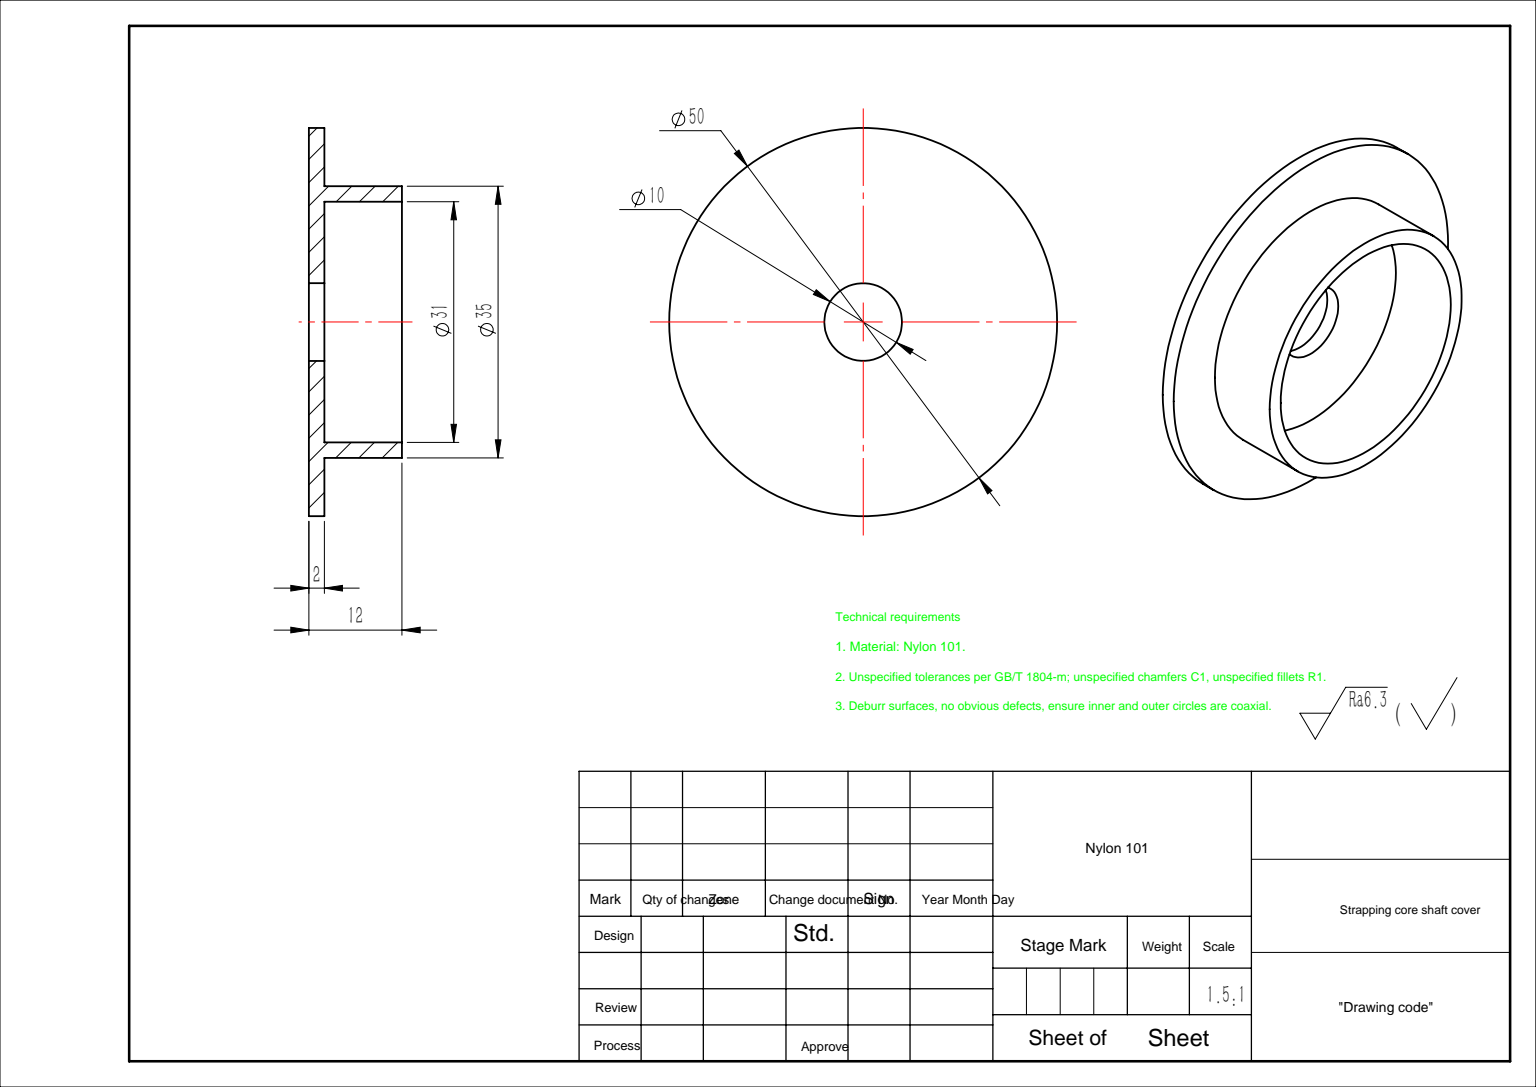
SolidWorks part; units mm, degrees
material "尼龙 101"
ref_plane "前视基准面" through (0, 0, 0) normal (0, 0, 1) x (1, 0, 0)
ref_plane "上视基准面" through (0, 0, 0) normal (0, 1, 0) x (1, 0, 0)
ref_plane "右视基准面" through (0, 0, 0) normal (1, 0, 0) x (0, 0, -1)
sketch "草图1" plane through (0, 0, 0) normal (0, 0, 1) x (1, 0, 0)
  line L0 (0, 30.304) -> (0, 0) construction
  line L1 (0, 0) -> (39.5369, 0) construction
  line L2 (0, 25) -> (2, 25)
  line L3 (2, 25) -> (2, 17.5)
  line L4 (2, 17.5) -> (12, 17.5)
  line L5 (12, 17.5) -> (12, 15.5)
  line L6 (12, 15.5) -> (2, 15.5)
  line L7 (2, 15.5) -> (2, 5)
  line L8 (2, 5) -> (0, 5)
  line L9 (0, 5) -> (0, 25)
  dimension "D1" = 10
  dimension "D2" = 50
  dimension "D3" = 2
  dimension "D4" = 2
  dimension "D5" = 7.5
  dimension "D6" = 10
revolve "旋转1" add sketch "草图1" angle 360 about L1
